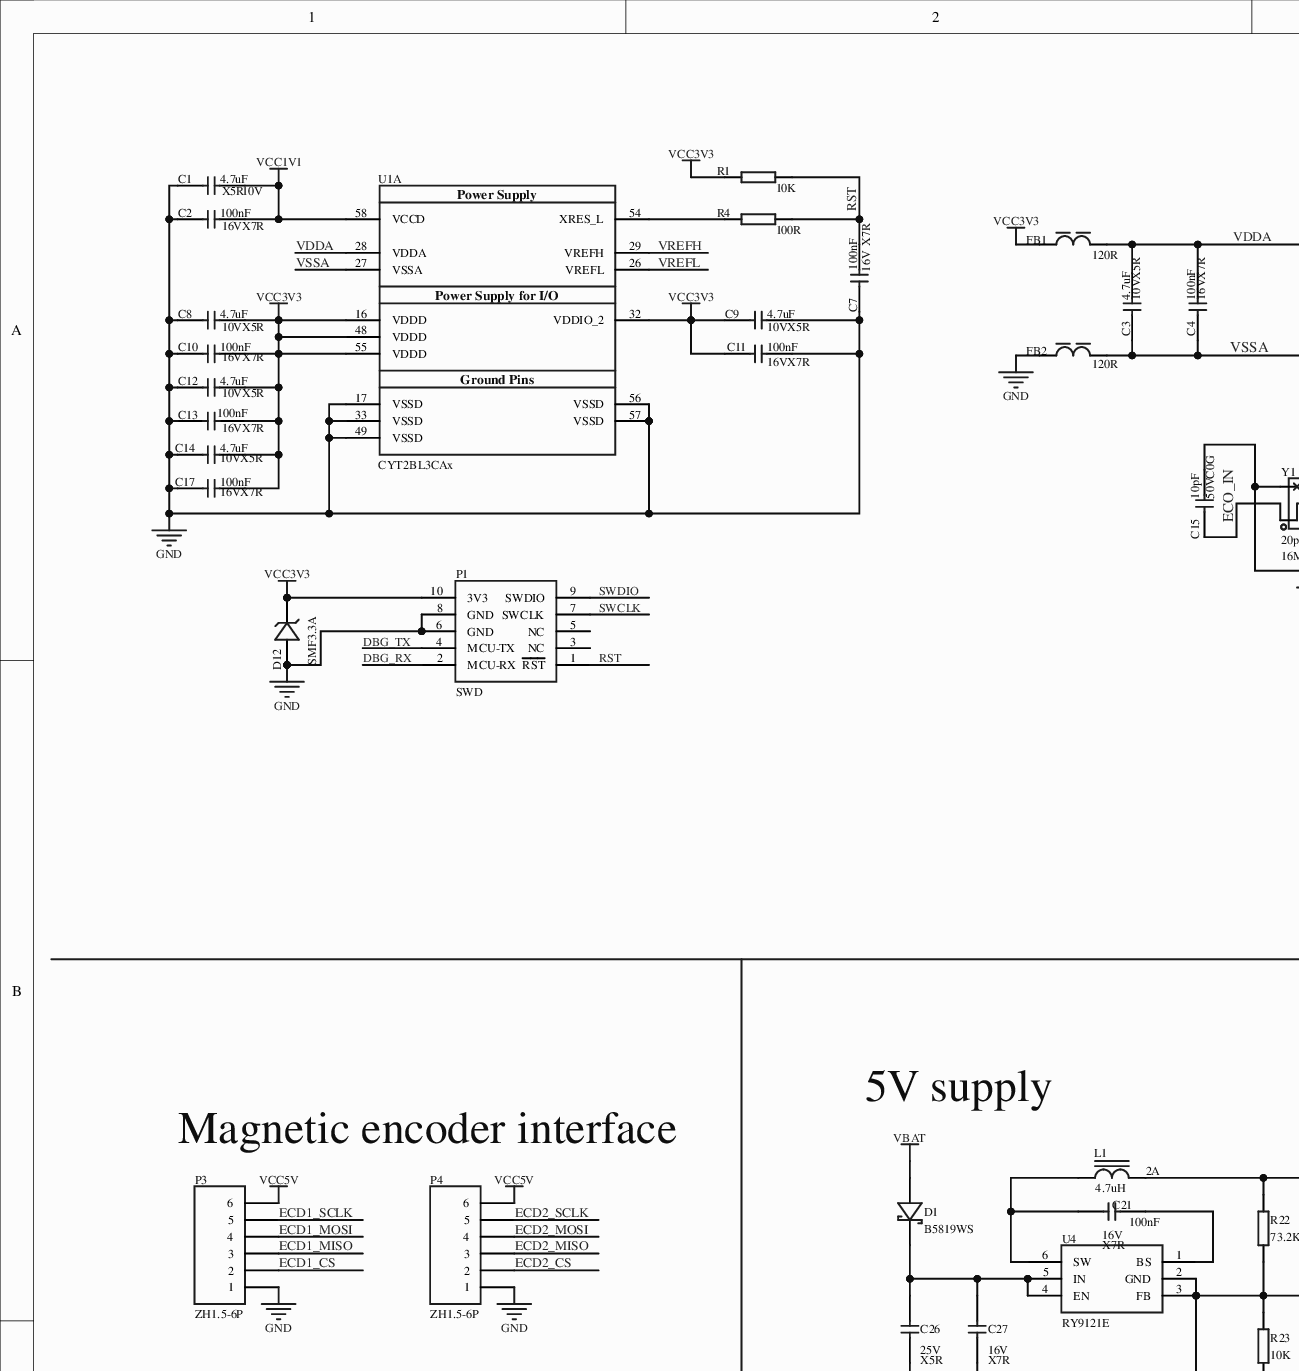
[diagram p0: MISC49862-3.schdoc, top left]
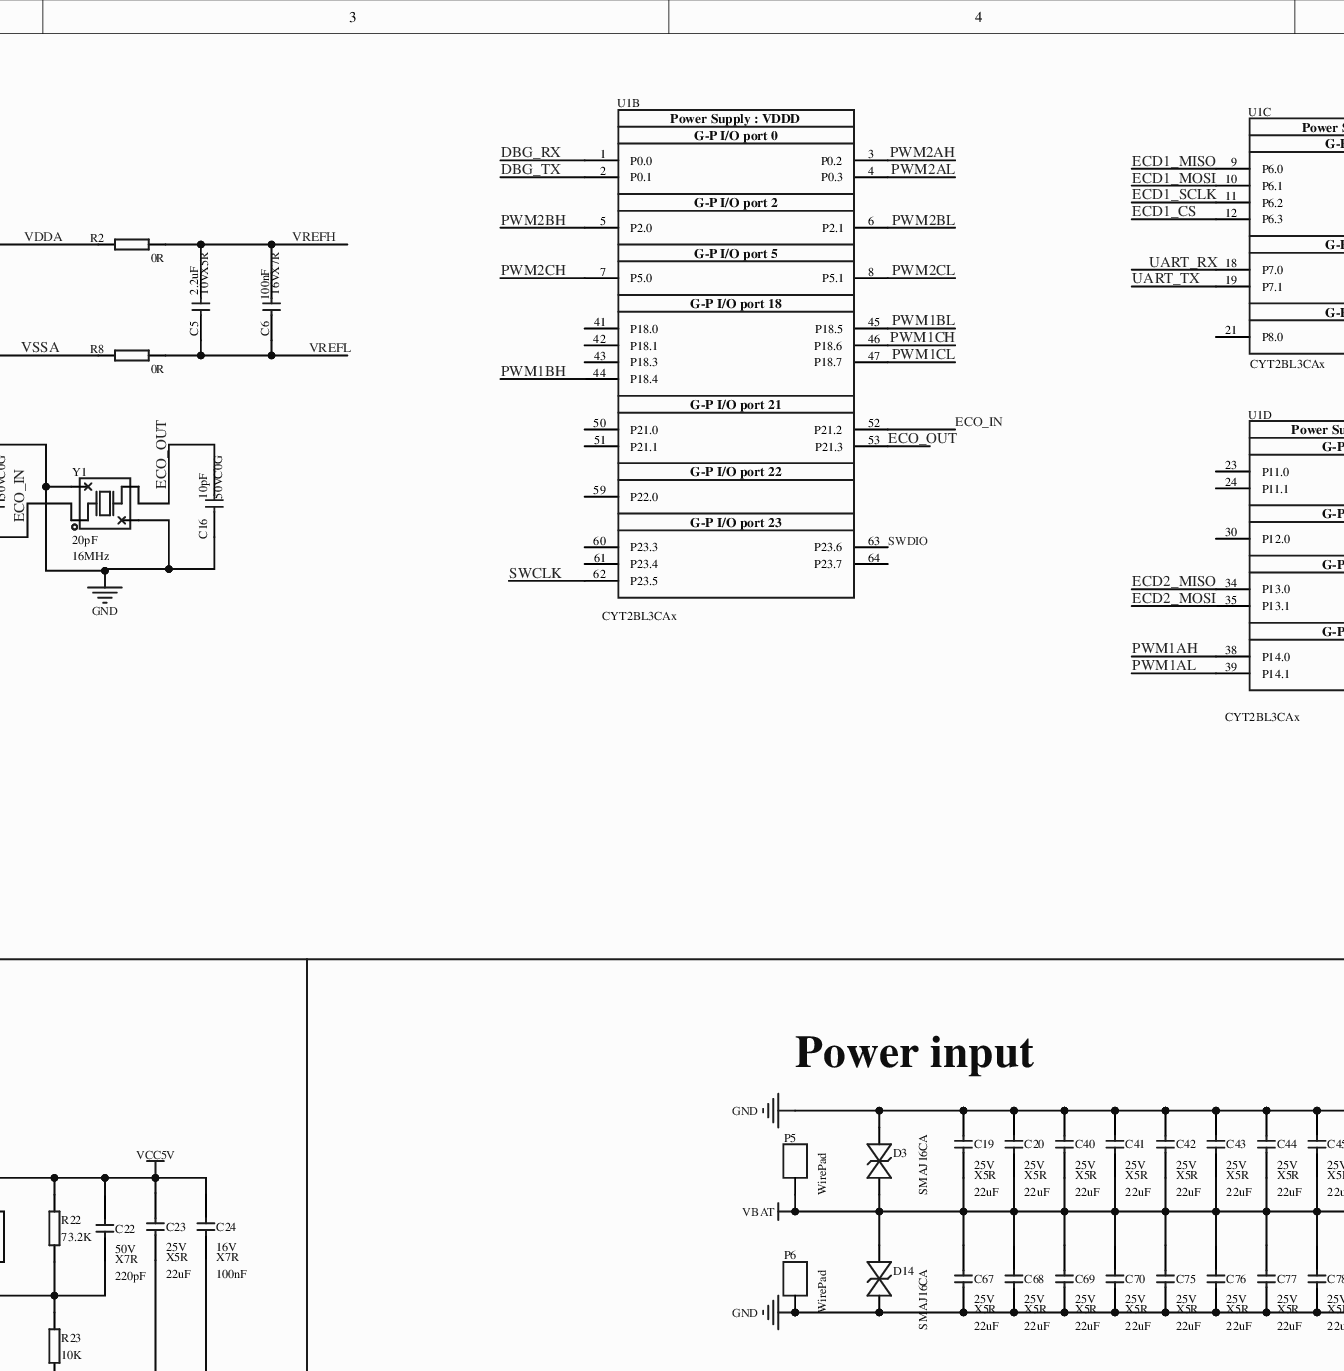
[diagram p1: MISC49862-3.schdoc, top middle]
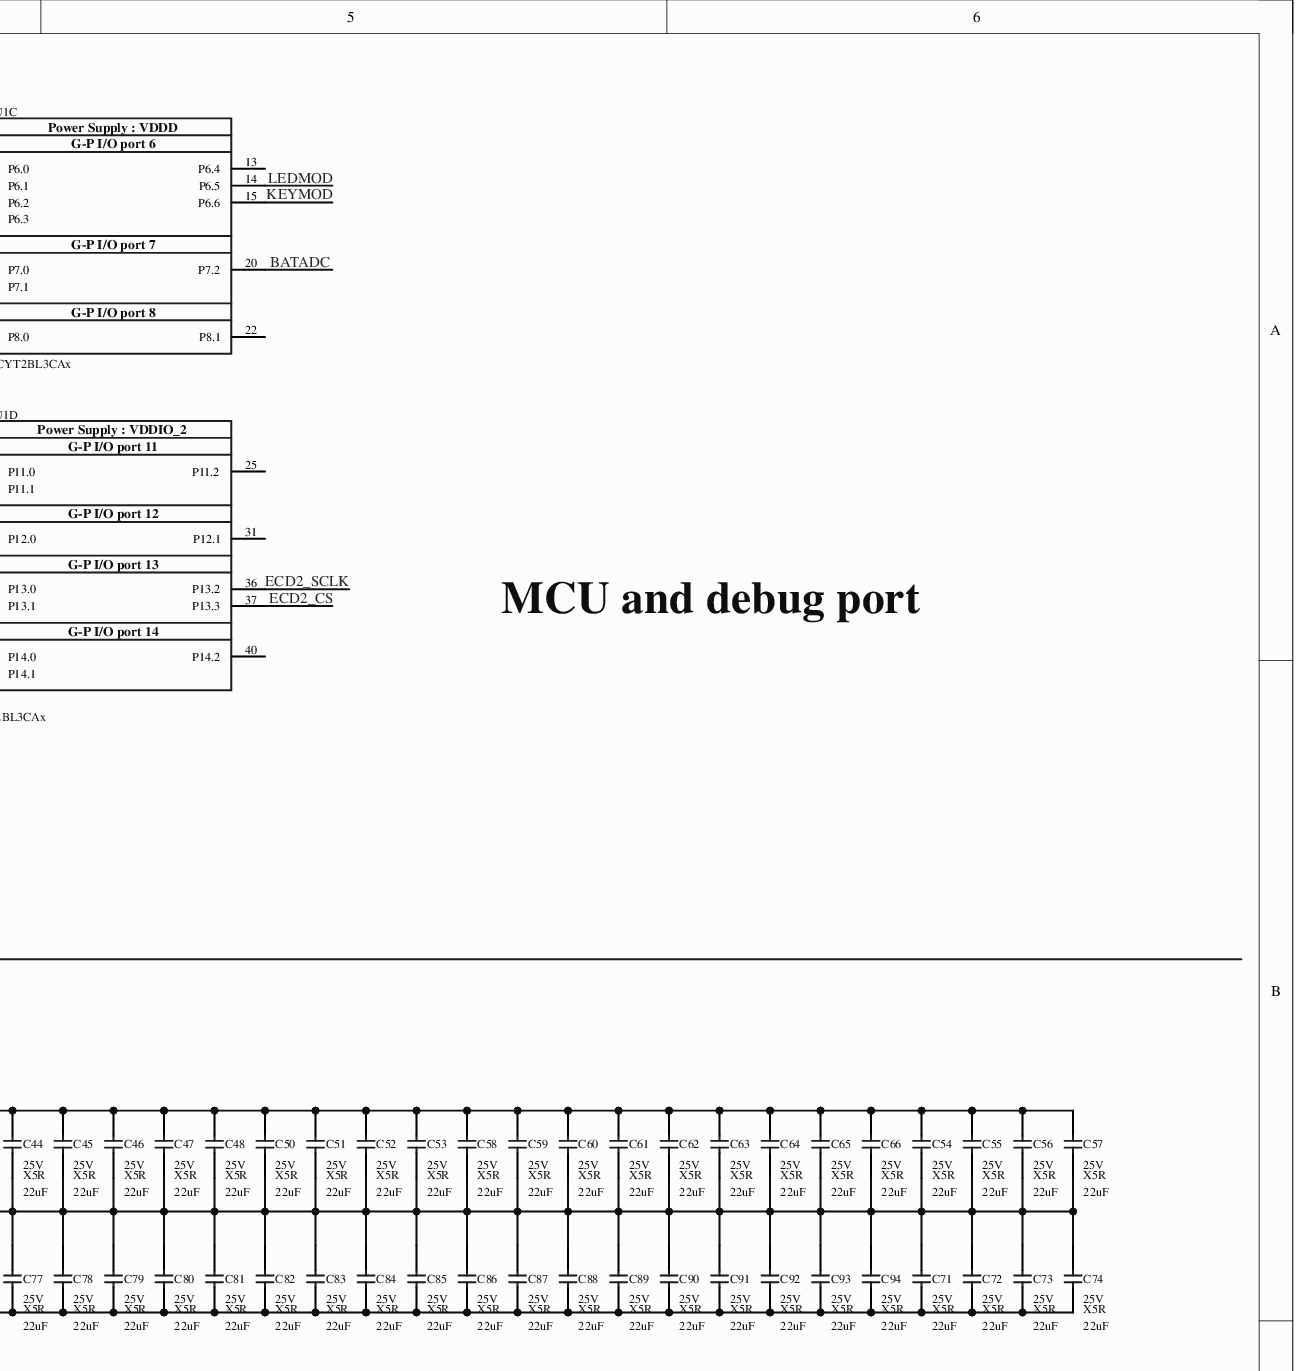
[diagram p2: MISC49862-3.schdoc, top right]
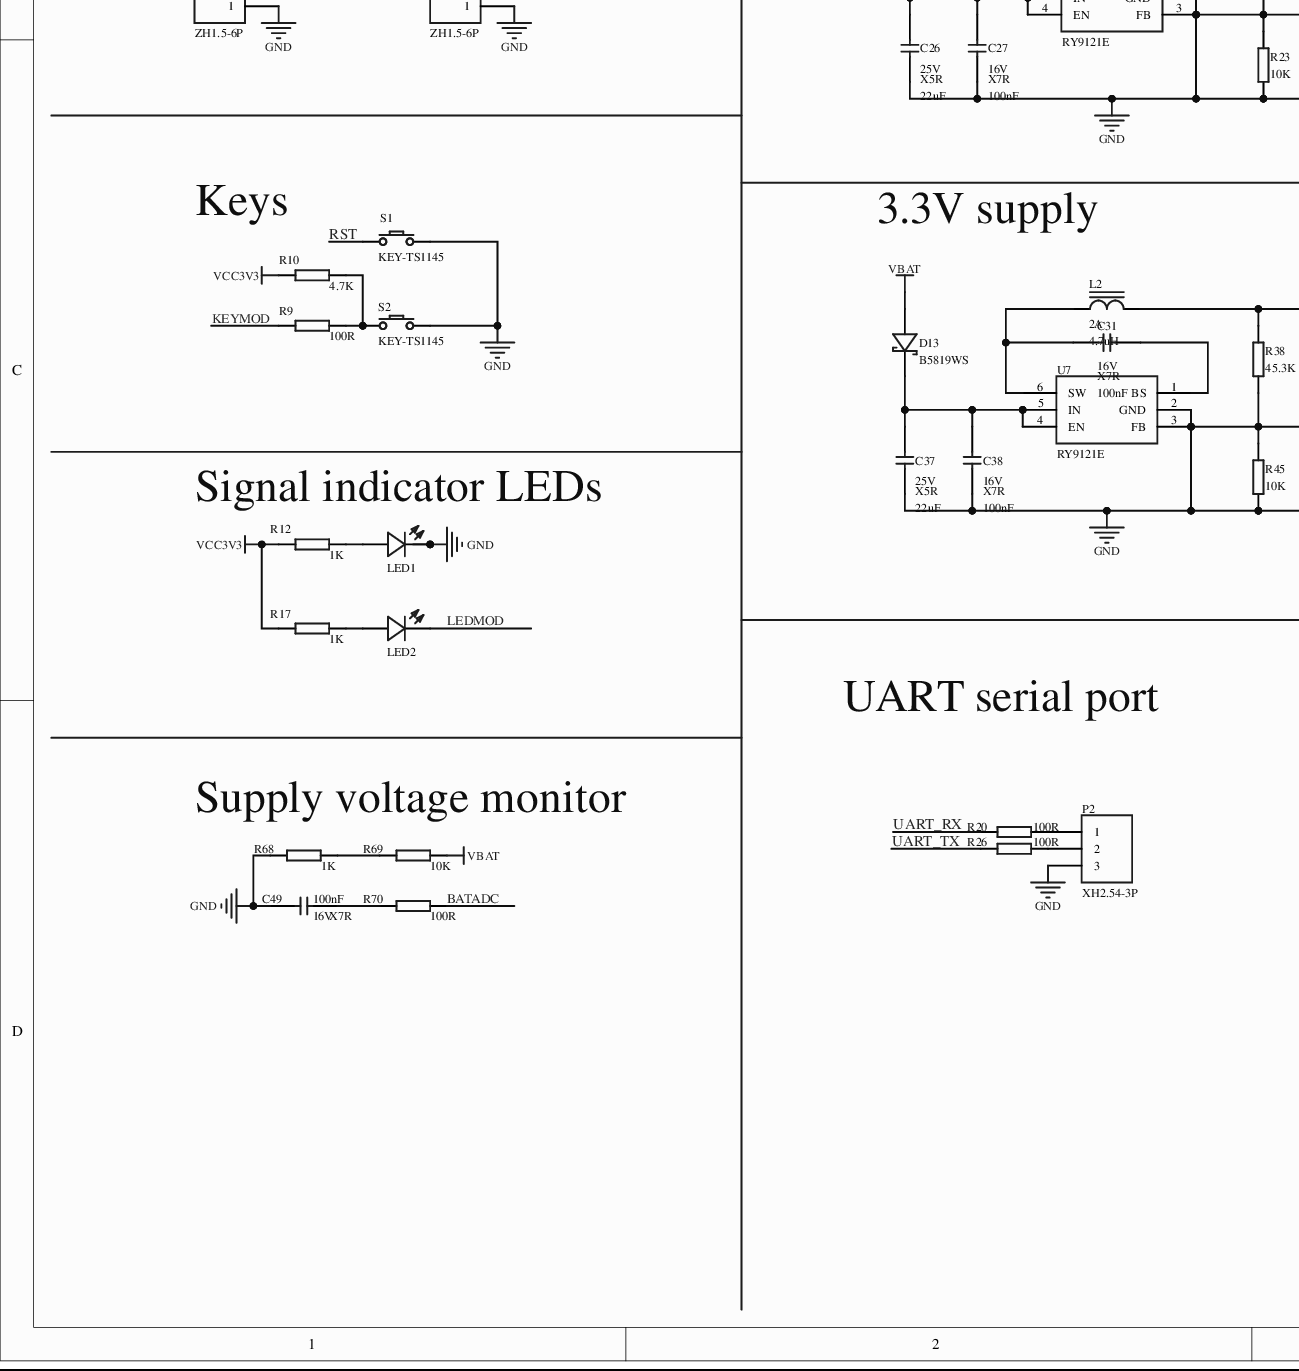
[diagram p3: MISC49862-3.schdoc, bottom left]
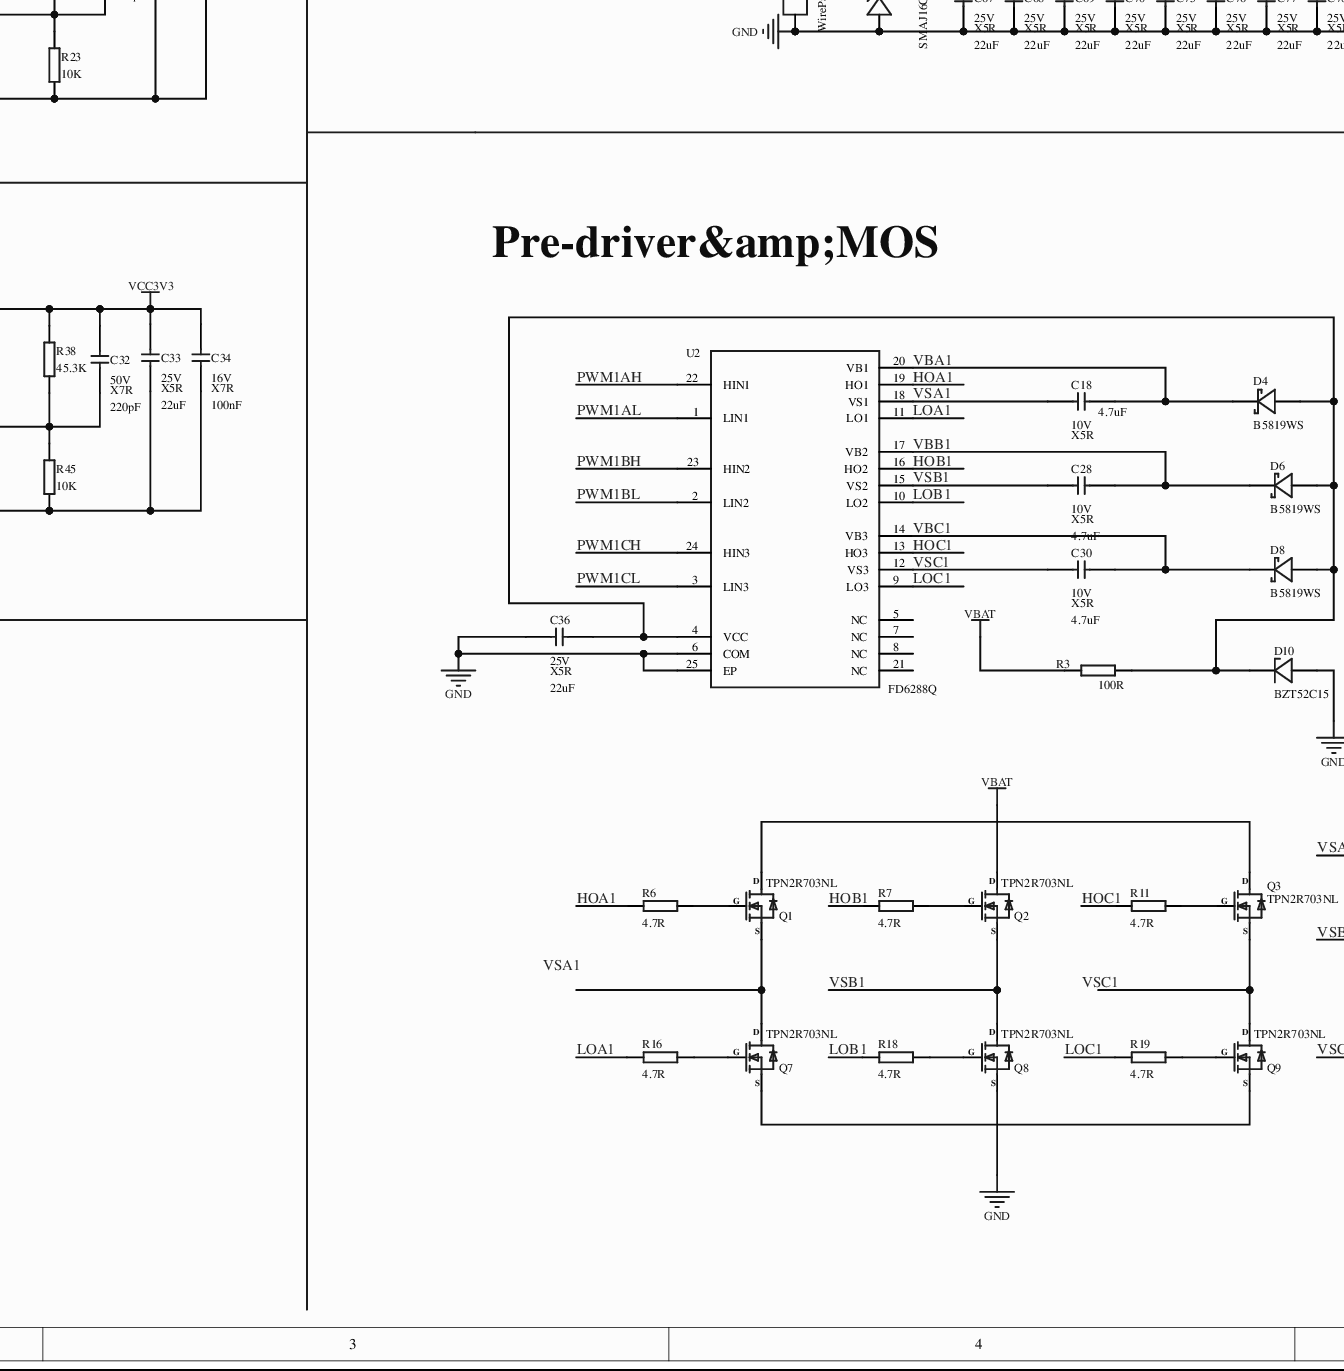
[diagram p4: MISC49862-3.schdoc, bottom middle]
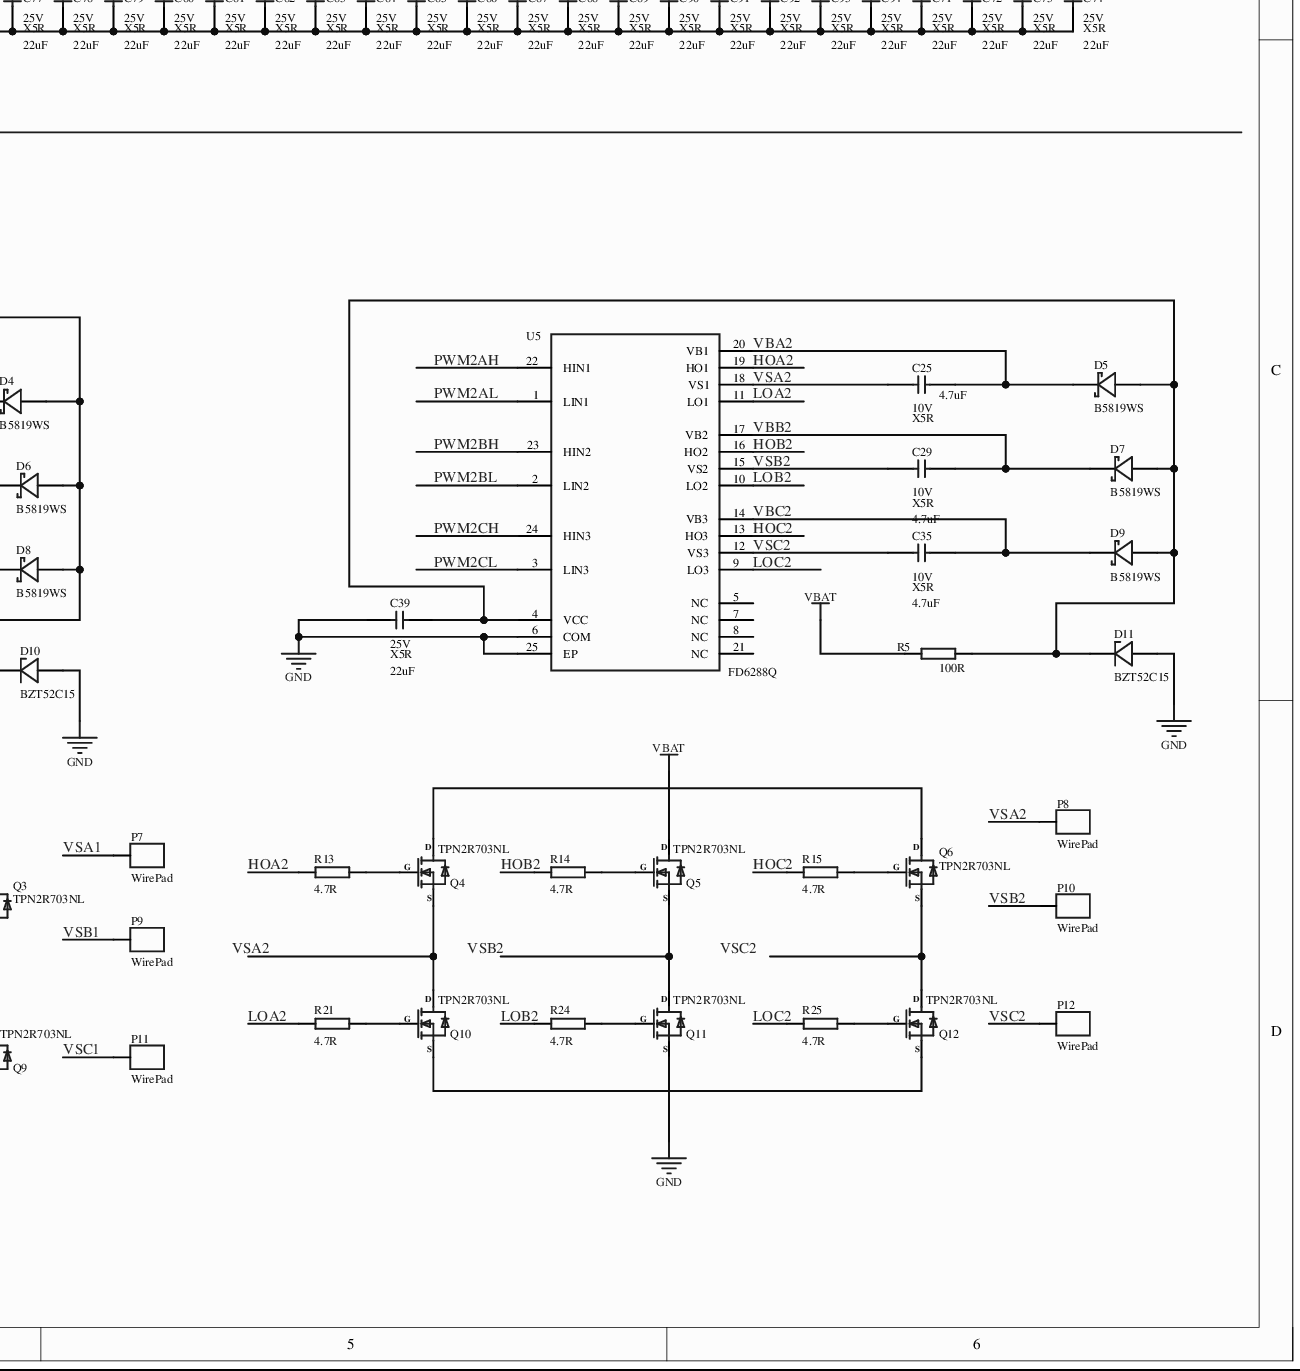
[diagram p5: MISC49862-3.schdoc, bottom right]
# Altium project MISC49862-2.PrjPcb (part 1 of 4)
1 sheet, 176 parts. Net scope: global (net labels, ports and power ports of the same name join across sheets).
Board file: MISC49862.pcbdoc

## Sheet MISC49862-3.schdoc
size 566 x 399 mm

### Parts
C1  value 4.7uF  Voltage: 10V  Type: X5R  [CAPC1005[0402]S-N]
C2  value 100nF  Voltage: 16V  Type: X7R  [CAPC1005[0402]S-N]
C3  value 4.7uF  Voltage: 10V  Type: X5R  [CAPC1005[0402]S-N]
C4  value 100nF  Voltage: 16V  Type: X7R  [CAPC1005[0402]S-N]
C5  value 2.2uF  Voltage: 10V  Type: X5R  [CAPC1005[0402]S-N]
C6  value 100nF  Voltage: 16V  Type: X7R  [CAPC1005[0402]S-N]
C7  value 100nF  Voltage: 16V  Type: X7R  [CAPC1005[0402]S-N]
C8  value 4.7uF  Voltage: 10V  Type: X5R  [CAPC1005[0402]S-N]
C9  value 4.7uF  Voltage: 10V  Type: X5R  [CAPC1005[0402]S-N]
C10  value 100nF  Voltage: 16V  Type: X7R  [CAPC1005[0402]S-N]
C11  value 100nF  Voltage: 16V  Type: X7R  [CAPC1005[0402]S-N]
C12  value 4.7uF  Voltage: 10V  Type: X5R  [CAPC1005[0402]S-N]
C13  value 100nF  Voltage: 16V  Type: X7R  [CAPC1005[0402]S-N]
C14  value 4.7uF  Voltage: 10V  Type: X5R  [CAPC1005[0402]S-N]
C15  value 10pF  Voltage: 50V  Type: C0G  [CAPC1005[0402]S-N]
C16  value 10pF  Voltage: 50V  Type: C0G  [CAPC1005[0402]S-N]
C17  value 100nF  Voltage: 16V  Type: X7R  [CAPC1005[0402]S-N]
C18  value 4.7uF  Voltage: 10V  Type: X5R  [CAPC1005[0402]S-N]
C19  value 22uF  Voltage: 25V  Type: X5R  [CAPC2012[0805]S-N]
C20  value 22uF  Voltage: 25V  Type: X5R  [CAPC2012[0805]S-N]
C21  value 100nF  Voltage: 16V  Type: X7R  [CAPC1005[0402]S-N]
C22  value 220pF  Voltage: 50V  Type: X7R  [CAPC1005[0402]S-N]
C23  value 22uF  Voltage: 25V  Type: X5R  [CAPC2012[0805]S-N]
C24  value 100nF  Voltage: 16V  Type: X7R  [CAPC1005[0402]S-N]
C25  value 4.7uF  Voltage: 10V  Type: X5R  [CAPC1005[0402]S-N]
C26  value 22uF  Voltage: 25V  Type: X5R  [CAPC2012[0805]S-N]
C27  value 100nF  Voltage: 16V  Type: X7R  [CAPC1005[0402]S-N]
C28  value 4.7uF  Voltage: 10V  Type: X5R  [CAPC1005[0402]S-N]
C29  value 4.7uF  Voltage: 10V  Type: X5R  [CAPC1005[0402]S-N]
C30  value 4.7uF  Voltage: 10V  Type: X5R  [CAPC1005[0402]S-N]
C31  value 100nF  Voltage: 16V  Type: X7R  [CAPC1005[0402]S-N]
C32  value 220pF  Voltage: 50V  Type: X7R  [CAPC1005[0402]S-N]
C33  value 22uF  Voltage: 25V  Type: X5R  [CAPC2012[0805]S-N]
C34  value 100nF  Voltage: 16V  Type: X7R  [CAPC1005[0402]S-N]
C35  value 4.7uF  Voltage: 10V  Type: X5R  [CAPC1005[0402]S-N]
C36  value 22uF  Voltage: 25V  Type: X5R  [CAPC2012[0805]S-N]
C37  value 22uF  Voltage: 25V  Type: X5R  [CAPC2012[0805]S-N]
C38  value 100nF  Voltage: 16V  Type: X7R  [CAPC1005[0402]S-N]
C39  value 22uF  Voltage: 25V  Type: X5R  [CAPC2012[0805]S-N]
C40  value 22uF  Voltage: 25V  Type: X5R  [CAPC2012[0805]S-N]
C41  value 22uF  Voltage: 25V  Type: X5R  [CAPC2012[0805]S-N]
C42  value 22uF  Voltage: 25V  Type: X5R  [CAPC2012[0805]S-N]
C43  value 22uF  Voltage: 25V  Type: X5R  [CAPC2012[0805]S-N]
C44  value 22uF  Voltage: 25V  Type: X5R  [CAPC2012[0805]S-N]
C45  value 22uF  Voltage: 25V  Type: X5R  [CAPC2012[0805]S-N]
C46  value 22uF  Voltage: 25V  Type: X5R  [CAPC2012[0805]S-N]
C47  value 22uF  Voltage: 25V  Type: X5R  [CAPC2012[0805]S-N]
C48  value 22uF  Voltage: 25V  Type: X5R  [CAPC2012[0805]S-N]
C49  value 100nF  Voltage: 16V  Type: X7R  [CAPC1005[0402]S-N]
C50  value 22uF  Voltage: 25V  Type: X5R  [CAPC2012[0805]S-N]
C51  value 22uF  Voltage: 25V  Type: X5R  [CAPC2012[0805]S-N]
C52  value 22uF  Voltage: 25V  Type: X5R  [CAPC2012[0805]S-N]
C53  value 22uF  Voltage: 25V  Type: X5R  [CAPC2012[0805]S-N]
C54  value 22uF  Voltage: 25V  Type: X5R  [CAPC2012[0805]S-N]
C55  value 22uF  Voltage: 25V  Type: X5R  [CAPC2012[0805]S-N]
C56  value 22uF  Voltage: 25V  Type: X5R  [CAPC2012[0805]S-N]
C57  value 22uF  Voltage: 25V  Type: X5R  [CAPC2012[0805]S-N]
C58  value 22uF  Voltage: 25V  Type: X5R  [CAPC2012[0805]S-N]
C59  value 22uF  Voltage: 25V  Type: X5R  [CAPC2012[0805]S-N]
C60  value 22uF  Voltage: 25V  Type: X5R  [CAPC2012[0805]S-N]
C61  value 22uF  Voltage: 25V  Type: X5R  [CAPC2012[0805]S-N]
C62  value 22uF  Voltage: 25V  Type: X5R  [CAPC2012[0805]S-N]
C63  value 22uF  Voltage: 25V  Type: X5R  [CAPC2012[0805]S-N]
C64  value 22uF  Voltage: 25V  Type: X5R  [CAPC2012[0805]S-N]
C65  value 22uF  Voltage: 25V  Type: X5R  [CAPC2012[0805]S-N]
C66  value 22uF  Voltage: 25V  Type: X5R  [CAPC2012[0805]S-N]
C67  value 22uF  Voltage: 25V  Type: X5R  [CAPC2012[0805]S-N]
C68  value 22uF  Voltage: 25V  Type: X5R  [CAPC2012[0805]S-N]
C69  value 22uF  Voltage: 25V  Type: X5R  [CAPC2012[0805]S-N]
C70  value 22uF  Voltage: 25V  Type: X5R  [CAPC2012[0805]S-N]
C71  value 22uF  Voltage: 25V  Type: X5R  [CAPC2012[0805]S-N]
C72  value 22uF  Voltage: 25V  Type: X5R  [CAPC2012[0805]S-N]
C73  value 22uF  Voltage: 25V  Type: X5R  [CAPC2012[0805]S-N]
C74  value 22uF  Voltage: 25V  Type: X5R  [CAPC2012[0805]S-N]
C75  value 22uF  Voltage: 25V  Type: X5R  [CAPC2012[0805]S-N]
C76  value 22uF  Voltage: 25V  Type: X5R  [CAPC2012[0805]S-N]
C77  value 22uF  Voltage: 25V  Type: X5R  [CAPC2012[0805]S-N]
C78  value 22uF  Voltage: 25V  Type: X5R  [CAPC2012[0805]S-N]
C79  value 22uF  Voltage: 25V  Type: X5R  [CAPC2012[0805]S-N]
C80  value 22uF  Voltage: 25V  Type: X5R  [CAPC2012[0805]S-N]
C81  value 22uF  Voltage: 25V  Type: X5R  [CAPC2012[0805]S-N]
C82  value 22uF  Voltage: 25V  Type: X5R  [CAPC2012[0805]S-N]
C83  value 22uF  Voltage: 25V  Type: X5R  [CAPC2012[0805]S-N]
C84  value 22uF  Voltage: 25V  Type: X5R  [CAPC2012[0805]S-N]
C85  value 22uF  Voltage: 25V  Type: X5R  [CAPC2012[0805]S-N]
C86  value 22uF  Voltage: 25V  Type: X5R  [CAPC2012[0805]S-N]
C87  value 22uF  Voltage: 25V  Type: X5R  [CAPC2012[0805]S-N]
C88  value 22uF  Voltage: 25V  Type: X5R  [CAPC2012[0805]S-N]
C89  value 22uF  Voltage: 25V  Type: X5R  [CAPC2012[0805]S-N]
C90  value 22uF  Voltage: 25V  Type: X5R  [CAPC2012[0805]S-N]
C91  value 22uF  Voltage: 25V  Type: X5R  [CAPC2012[0805]S-N]
C92  value 22uF  Voltage: 25V  Type: X5R  [CAPC2012[0805]S-N]
C93  value 22uF  Voltage: 25V  Type: X5R  [CAPC2012[0805]S-N]
C94  value 22uF  Voltage: 25V  Type: X5R  [CAPC2012[0805]S-N]
D1  B5819WS  [SOD-323]
D3  SMAJ16CA  [SMA[DO-214AC]-Bi]
D4  B5819WS  [SOD-323]
D5  B5819WS  [SOD-323]
D6  B5819WS  [SOD-323]
D7  B5819WS  [SOD-323]
D8  B5819WS  [SOD-323]
D9  B5819WS  [SOD-323]
D10  BZT52C15  [SOD-123-L]
D11  BZT52C15  [SOD-123-L]
D12  SMF3.3A  [SOD-123-FL]
D13  B5819WS  [SOD-323]
D14  SMAJ16CA  [SMA[DO-214AC]-Bi]
FB1  value 120R  [INDC1005[0402]S]
FB2  value 120R  [INDC1005[0402]S]
L1  value 4.7uH  Imax: 2A  [SLO2520]
L2  value 4.7uH  Imax: 2A  [SLO2520]
LED1  Red SMD LED  [LEDC1608(0603)-L]  (value not drawn)
LED2  Blue SMD LED  [LEDC1608(0603)-L]  (value not drawn)
P1  value SWD  [HDR2X5-OB]  (hidden comment: SWD Header 5x2)
P2  XH2.54-3P  [XH2.54-3P-SH]
P3  ZH1.5-6P  [ZH1.5-6P-SH]
P4  ZH1.5-6P  [ZH1.5-6P-SH]
P5  WirePad  [WirePad-4x6]
P6  WirePad  [WirePad-4x6]
P7  WirePad  [WirePad-4x6]
P8  WirePad  [WirePad-4x6]
P9  WirePad  [WirePad-4x6]
P10  WirePad  [WirePad-4x6]
P11  WirePad  [WirePad-4x6]
P12  WirePad  [WirePad-4x6]
Q1  TPN2R703NL  [TSON3x3]
Q2  TPN2R703NL  [TSON3x3]
Q3  TPN2R703NL  [TSON3x3]
Q4  TPN2R703NL  [TSON3x3]
Q5  TPN2R703NL  [TSON3x3]
Q6  TPN2R703NL  [TSON3x3]
Q7  TPN2R703NL  [TSON3x3]
Q8  TPN2R703NL  [TSON3x3]
Q9  TPN2R703NL  [TSON3x3]
Q10  TPN2R703NL  [TSON3x3]
Q11  TPN2R703NL  [TSON3x3]
Q12  TPN2R703NL  [TSON3x3]
R1  value 10K  [RESC1005[0402]S-N]
R2  value 0R  [RESC1005[0402]S-N]
R3  value 100R  [RESC1005[0402]S-N]
R4  value 100R  [RESC1005[0402]S-N]
R5  value 100R  [RESC1005[0402]S-N]
R6  value 4.7R  [RESC1005[0402]S-N]
R7  value 4.7R  [RESC1005[0402]S-N]
R8  value 0R  [RESC1005[0402]S-N]
R9  value 100R  [RESC1005[0402]S-N]
R10  value 4.7K  [RESC1005[0402]S-N]
R11  value 4.7R  [RESC1005[0402]S-N]
R12  value 1K  [RESC1005[0402]S-N]
R13  value 4.7R  [RESC1005[0402]S-N]
R14  value 4.7R  [RESC1005[0402]S-N]
R15  value 4.7R  [RESC1005[0402]S-N]
R16  value 4.7R  [RESC1005[0402]S-N]
R17  value 1K  [RESC1005[0402]S-N]
R18  value 4.7R  [RESC1005[0402]S-N]
R19  value 4.7R  [RESC1005[0402]S-N]
R20  value 100R  [RESC1005[0402]S-N]
R21  value 4.7R  [RESC1005[0402]S-N]
R22  value 73.2K  [RESC1005[0402]S-N]
R23  value 10K  [RESC1005[0402]S-N]
R24  value 4.7R  [RESC1005[0402]S-N]
R25  value 4.7R  [RESC1005[0402]S-N]
R26  value 100R  [RESC1005[0402]S-N]
R38  value 45.3K  [RESC1005[0402]S-N]
R45  value 10K  [RESC1005[0402]S-N]
R68  value 1K  [RESC1005[0402]S-N]
R69  value 10K  [RESC1005[0402]S-N]
R70  value 100R  [RESC1005[0402]S-N]
S1  KEY-TS1145  [TS1145-B-A]
S2  KEY-TS1145  [TS1145-B-A]
U1  CYT2BL3CAx  [LQFP64_L]  (parts A,B,C,D of 4)
U2  FD6288Q  [QFN24-4x4-L]
U4  RY9121E  [SOT-23-6]
U5  FD6288Q  [QFN24-4x4-L]
U7  RY9121E  [SOT-23-6]
Y1  Load_Capactiance: 20pF  Frequency: 16MHz  [X3225-4]

### Nets
GND: C1.1 C2.1 C7.1 C8.1 C9.2 C10.1 C11.2 C12.1 C13.1 C14.1 C15.2 C16.1 C17.1 C19.2 C20.2 C22.1 C23.1 C24.1 C26.1 C27.1 C32.1 C33.1 C34.1 C36.2 C37.1 C38.1 C39.2 C40.2 C41.2 C42.2 C43.2 C44.2 C45.2 C46.2 C47.2 C48.2 C49.1 C50.2 C51.2 C52.2 C53.2 C54.2 C55.2 C56.2 C57.2 C58.2 C59.2 C60.2 C61.2 C62.2 C63.2 C64.2 C65.2 C66.2 C67.1 C68.1 C69.1 C70.1 C71.1 C72.1 C73.1 C74.1 C75.1 C76.1 C77.1 C78.1 C79.1 C80.1 C81.1 C82.1 C83.1 C84.1 C85.1 C86.1 C87.1 C88.1 C89.1 C90.1 C91.1 C92.1 C93.1 C94.1 D3.K D10.A D11.A D12.A D14.A FB2.1 LED1.C P1.6(GND) P1.8(GND) P2.3 P3.1 P4.1 P6.1 Q8.3(S) Q11.3(S) R22.1 R23.1 R23.2 R38.1 R45.1 R45.2 R68.1 S1.1 S2.1 U1.17(VSSD) U1.33(VSSD) U1.49(VSSD) U1.56(VSSD) U1.57(VSSD) U2.6(COM) U2.25(EP) U4.2(GND) U4.3(FB) U5.6(COM) U5.25(EP) U7.2(GND) U7.3(FB) Y1.2(NC) Y1.4(NC)
VBAT: C19.1 C20.1 C40.1 C41.1 C42.1 C43.1 C44.1 C45.1 C46.1 C47.1 C48.1 C50.1 C51.1 C52.1 C53.1 C54.1 C55.1 C56.1 C57.1 C58.1 C59.1 C60.1 C61.1 C62.1 C63.1 C64.1 C65.1 C66.1 C67.2 C68.2 C69.2 C70.2 C71.2 C72.2 C73.2 C74.2 C75.2 C76.2 C77.2 C78.2 C79.2 C80.2 C81.2 C82.2 C83.2 C84.2 C85.2 C86.2 C87.2 C88.2 C89.2 C90.2 C91.2 C92.2 C93.2 C94.2 D1.A D3.A D13.A D14.K P5.1 Q2.1(D) Q5.1(D) R3.1 R5.1 R69.2
VCC1V1: C1.2 C2.2 U1.58(VCCD)
VCC3V3: C8.2 C9.1 C10.2 C11.1 C12.2 C13.2 C14.2 C17.2 C32.2 C33.2 C34.2 D12.K FB1.1 L2.1 P1.10(3V3) R1.1 R10.1 R12.1 R17.1 R38.2 U1.16(VDDD) U1.32(VDDIO_2) U1.48(VDDD) U1.55(VDDD)
VCC5V: C22.2 C23.2 C24.2 L1.1 P3.6 P4.6 R22.2
BATADC: R70.2 U1.20(P7.2)
DBG_RX: P1.2(MCU-RX) U1.1(P0.0)
DBG_TX: P1.4(MCU-TX) U1.2(P0.1)
ECD1_CS: P3.2 U1.12(P6.3)
ECD1_MISO: P3.3 U1.9(P6.0)
ECD1_MOSI: P3.4 U1.10(P6.1)
ECD1_SCLK: P3.5 U1.11(P6.2)
ECD2_CS: P4.2 U1.37(P13.3)
ECD2_MISO: P4.3 U1.34(P13.0)
ECD2_MOSI: P4.4 U1.35(P13.1)
ECD2_SCLK: P4.5 U1.36(P13.2)
ECO_IN: C15.1 U1.52(P21.2) Y1.1(OSC1)
ECO_OUT: C16.2 U1.53(P21.3) Y1.3(OSC2)
HOA1: R6.1 U2.19(HO1)
HOA2: R13.1 U5.19(HO1)
HOB1: R7.1 U2.16(HO2)
HOB2: R14.1 U5.16(HO2)
HOC1: R11.1 U2.13(HO3)
HOC2: R15.1 U5.13(HO3)
KEYMOD: R9.1 U1.15(P6.6)
LEDMOD: LED2.C U1.14(P6.5)
LOA1: R16.1 U2.11(LO1)
LOA2: R21.1 U5.11(LO1)
LOB1: R18.1 U2.10(LO2)
LOB2: R24.1 U5.10(LO2)
LOC1: R19.1 U2.9(LO3)
LOC2: R25.1 U5.9(LO3)
PWM1AH: U1.38(P14.0) U2.22(HIN1)
PWM1AL: U1.39(P14.1) U2.1(LIN1)
PWM1BH: U1.44(P18.4) U2.23(HIN2)
PWM1BL: U1.45(P18.5) U2.2(LIN2)
PWM1CH: U1.46(P18.6) U2.24(HIN3)
PWM1CL: U1.47(P18.7) U2.3(LIN3)
PWM2AH: U1.3(P0.2) U5.22(HIN1)
PWM2AL: U1.4(P0.3) U5.1(LIN1)
PWM2BH: U1.5(P2.0) U5.23(HIN2)
PWM2BL: U1.6(P2.1) U5.2(LIN2)
PWM2CH: U1.7(P5.0) U5.24(HIN3)
PWM2CL: U1.8(P5.1) U5.3(LIN3)
RST: C7.2 P1.1(~{RST}) R1.2 R4.2 S1.2
SWCLK: P1.7(SWCLK) U1.62(P23.5)
SWDIO: P1.9(SWDIO) U1.63(P23.6)
UART_RX: R20.1 U1.18(P7.0)
UART_TX: R26.1 U1.19(P7.1)
VBA1: C18.2 D4.K U2.20(VB1)
VBA2: C25.2 D5.K U5.20(VB1)
VBB1: C28.2 D6.K U2.17(VB2)
VBB2: C29.2 D7.K U5.17(VB2)
VBC1: C30.2 D8.K U2.14(VB3)
VBC2: C35.2 D9.K U5.14(VB3)
VDDA: C3.1 C4.2 FB1.2 R2.1 U1.28(VDDA)
VREFH: C5.2 C6.2 R2.2 U1.29(VREFH)
VREFL: C5.1 C6.1 R8.2 U1.26(VREFL)
VSA1: C18.1 P7.1 U2.18(VS1)
VSA2: C25.1 P8.1 U5.18(VS1)
VSB1: C28.1 P9.1 Q2.3(S) Q8.1(D) U2.15(VS2)
VSB2: C29.1 P10.1 U5.15(VS2)
VSC1: C30.1 P11.1 U2.12(VS3)
VSC2: C35.1 P12.1 U5.12(VS3)
VSSA: C3.2 C4.1 FB2.2 R8.1 U1.27(VSSA)
NetC21_1: C21.1 U4.1(BS)
NetC21_2: C21.2 L1.2 U4.6(SW)
NetC26_2: C26.2 C27.2 D1.K U4.4(EN) U4.5(IN)
NetC31_1: C31.1 U7.1(BS)
NetC31_2: C31.2 L2.2 U7.6(SW)
NetC36_1: C36.1 D4.A D6.A D8.A D10.K R3.2 U2.4(VCC)
NetC37_2: C37.2 C38.2 D13.K U7.4(EN) U7.5(IN)
NetC39_1: C39.1 D5.A D7.A D9.A D11.K R5.2 U5.4(VCC)
NetC49_2: C49.2 R70.1
NetLED1_A: LED1.A R12.2
NetLED2_A: LED2.A R17.2
NetP2_1: P2.1 R20.2
NetP2_2: P2.2 R26.2
NetQ1_1: Q1.1(D) Q3.1(D)
NetQ1_2: Q1.2(G) R6.2
NetQ1_3: Q1.3(S) Q7.1(D)
NetQ2_2: Q2.2(G) R7.2
NetQ3_2: Q3.2(G) R11.2
NetQ3_3: Q3.3(S) Q9.1(D)
NetQ4_1: Q4.1(D) Q6.1(D)
NetQ4_2: Q4.2(G) R13.2
NetQ4_3: Q4.3(S) Q10.1(D)
NetQ5_2: Q5.2(G) R14.2
NetQ5_3: Q5.3(S) Q11.1(D)
NetQ6_2: Q6.2(G) R15.2
NetQ6_3: Q6.3(S) Q12.1(D)
NetQ7_2: Q7.2(G) R16.2
NetQ7_3: Q7.3(S) Q9.3(S)
NetQ8_2: Q8.2(G) R18.2
NetQ9_2: Q9.2(G) R19.2
NetQ10_2: Q10.2(G) R21.2
NetQ10_3: Q10.3(S) Q12.3(S)
NetQ11_2: Q11.2(G) R24.2
NetQ12_2: Q12.2(G) R25.2
NetR4_1: R4.1 U1.54(XRES_L)
NetR9_2: R9.2 R10.2 S2.2
NetR68_2: R68.2 R69.1

Not connected (* = marked no-connect by the designer): P1 3(NC)* 5(NC)*; U1 13(P6.4) 21(P8.0) 22(P8.1) 23(P11.0) 24(P11.1) 25(P11.2) 30(P12.0) 31(P12.1) 40(P14.2) 41(P18.0) 42(P18.1) 43(P18.3) 50(P21.0) 51(P21.1) 59(P22.0) 60(P23.3) 61(P23.4) 64(P23.7); U2 5(NC)* 7(NC)* 8(NC)* 21(NC)*; U5 5(NC)* 7(NC)* 8(NC)* 21(NC)*

### Notes on the sheet
- MCU and debug port
- Power input
- Magnetic encoder interface
- 5V supply
- (near R10) Keys
- Pre-driver&amp;MOS
- 3.3V supply
- Signal indicator LEDs
- UART serial port
- Supply voltage monitor
- Labels drawn without touching a wire or pin: VSA1, VSA2, VSB2, VSC1, VSC2